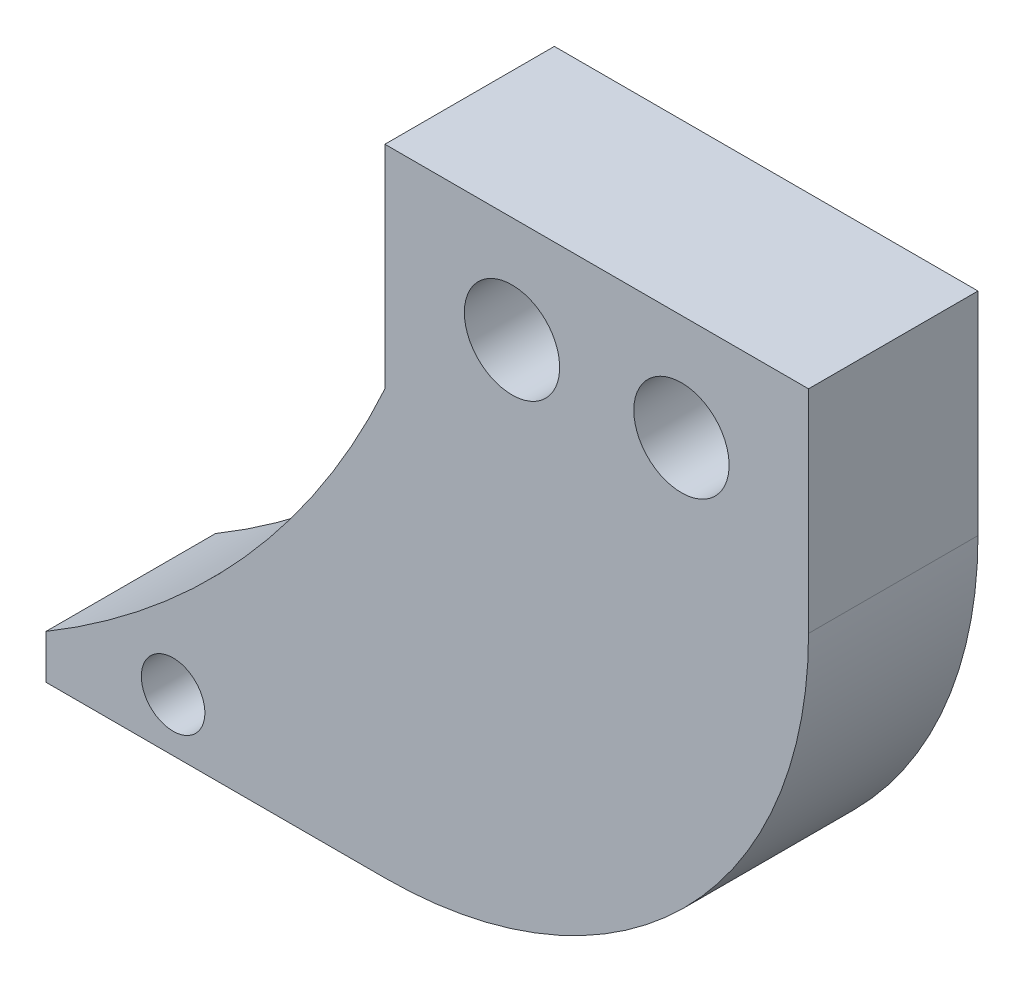
SolidWorks part; units mm, degrees
ref_plane "前视基准面" through (0, 0, 0) normal (0, 0, 1) x (1, 0, 0)
ref_plane "上视基准面" through (0, 0, 0) normal (0, 1, 0) x (1, 0, 0)
ref_plane "右视基准面" through (0, 0, 0) normal (1, 0, 0) x (0, 0, -1)
sketch "草图1" plane through (0, 0, 0) normal (0, 0, 1) x (1, 0, 0)
  line L1 (-6.6805, 8.5685) -> (13.3195, 8.5685)
  line L2 (-6.6805, 8.5685) -> (-6.6805, -1.4315)
  line L4 (13.3195, 8.5685) -> (13.3195, -1.4315)
  line L5 (-6.6805, -21.4315) -> (-22.6805, -21.4315)
  line L6 (-22.6805, -21.4315) -> (-22.6805, -19.3495)
  arc A0 (-6.6805, -21.4315) -> (13.3195, -1.4315) centre (-6.6805, -1.4315) ccw
  arc A2 (-22.6805, -19.3495) -> (-6.6805, -1.4315) centre (-43.0905, 14.9785) ccw
  dimension "D1" = 20
  dimension "D2" = 10
  dimension "D3" = 36.41
  dimension "D4" = 6.41
  dimension "D6" = 16
extrude "凸台-拉伸1" add sketch "草图1" along normal blind 8
sketch "草图2" plane through (0, 0, 0) normal (0, 0, -1) x (-1, 0, 0)
  line L0 (-13.3195, 8.5685) -> (6.6805, 8.5685) construction
  line L1 (6.6805, 8.5685) -> (6.6805, -1.4315) construction
  line L2 (-13.3195, -1.4315) -> (-13.3195, 8.5685) construction
  line L3 (22.6805, -21.4315) -> (6.6805, -21.4315) construction
  line L4 (22.6805, -19.3495) -> (22.6805, -21.4315) construction
  circle A0 centre (16.6805, -18.9315) radius 1.5
  circle A1 centre (0.6805, 3.5685) radius 2.25
  circle A2 centre (-7.3195, 3.5685) radius 2.25
  dimension "D5" = 4.5
  dimension "D6" = 4.5
  dimension "D9" = 3
  dimension "D1" = 5
  dimension "D2" = 6
  dimension "D3" = 5
  dimension "D4" = 6
  dimension "D7" = 2.5
  dimension "D8" = 6
extrude "切除-拉伸1" cut sketch "草图2" against normal through all
